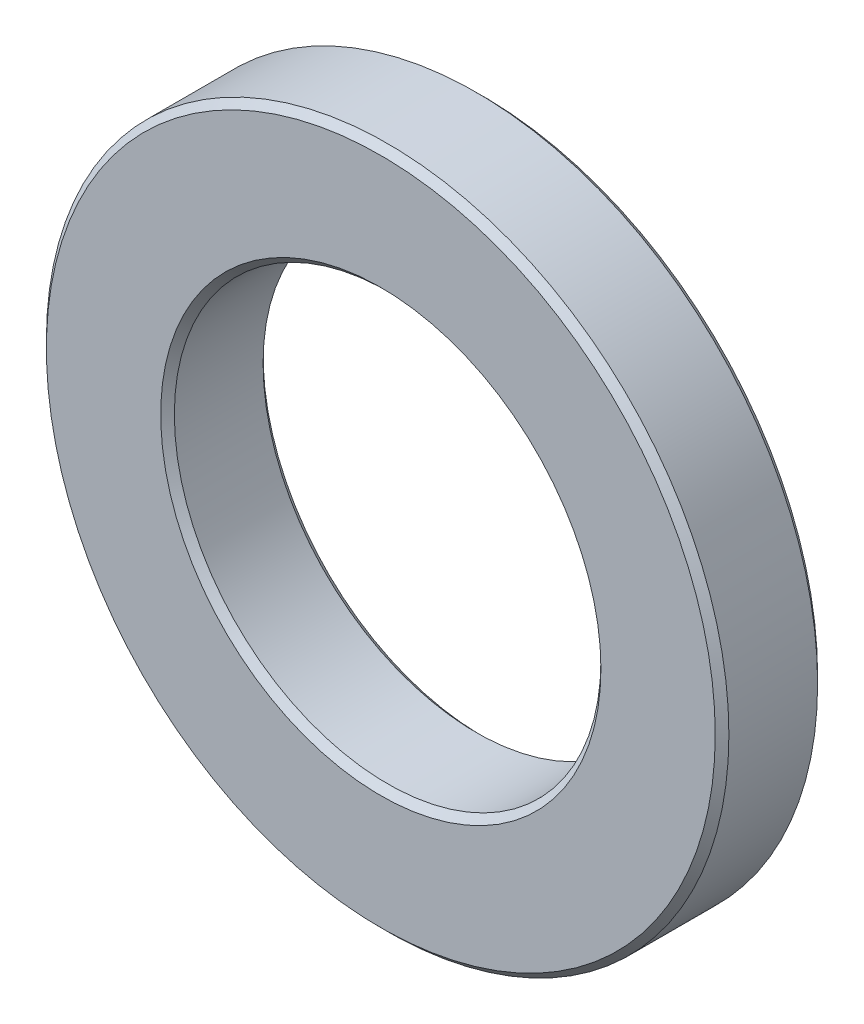
SolidWorks part; units mm, degrees
ref_plane "Front Plane" through (0, 0, 0) normal (0, 0, 1) x (1, 0, 0)
ref_plane "Top Plane" through (0, 0, 0) normal (0, 1, 0) x (1, 0, 0)
ref_plane "Right Plane" through (0, 0, 0) normal (1, 0, 0) x (0, 0, -1)
sketch "Sketch1" plane through (0, 0, 0) normal (0, 0, 1) x (1, 0, 0)
  circle A0 centre (0, 0) radius 10
  circle A1 centre (0, 0) radius 6.25
  dimension "D1" = 12.5
  dimension "D2" = 20
extrude "Boss-Extrude1" add sketch "Sketch1" along normal blind 3
chamfer "Chamfer1" distance 0.2 angle 45 4 edges at (6.25, 0, 0) (10, 0, 0) (6.25, 0, 3) (10, 0, 3)
